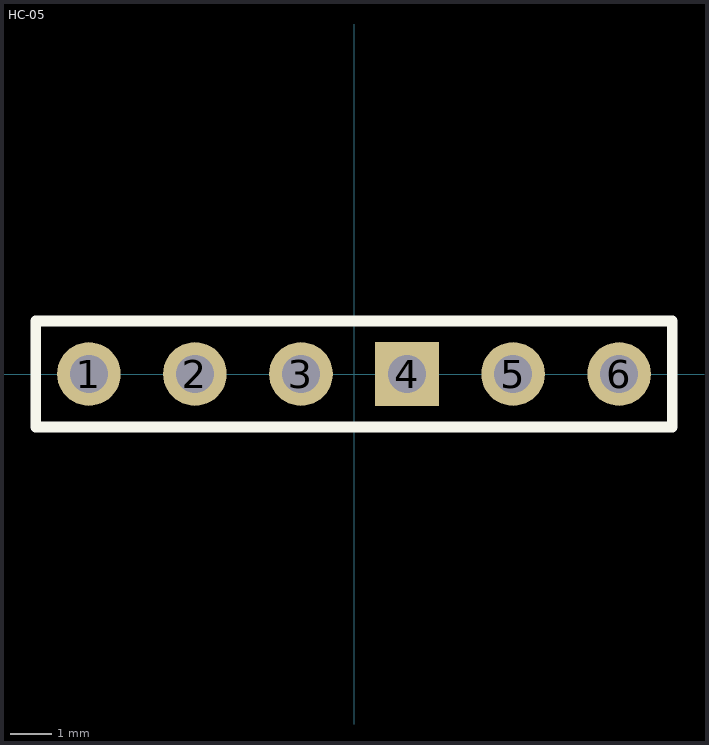
[diagram p0: the footprint, top view; thin cyan lines are the x and y axes]
# Altium footprint library MISC84237-9.PcbLib: 1 footprints
Each footprint in its own frame and in the unit in brackets; x right, y up, seen from the top. Pads: shape width x height; smd on the part's side, far side on the other; paste and mask are expansions set on the pad; w line width, h text height; cw(c..) or ccw(c..) is an arc to the next point about the centre after c.

## HC-05 [mil]
pads (6):
  round 60 hole 36 paste+4 mask+4: 1(-250,0) 2(-150,0) 3(-50,0) 5(150,0) 6(250,0)
  rect 60x60 hole 36 paste+4 mask+4: 4(50,0)
Top Overlay:
  lines w10: -300,-50 -300,50 300,50 300,-50 -300,-50